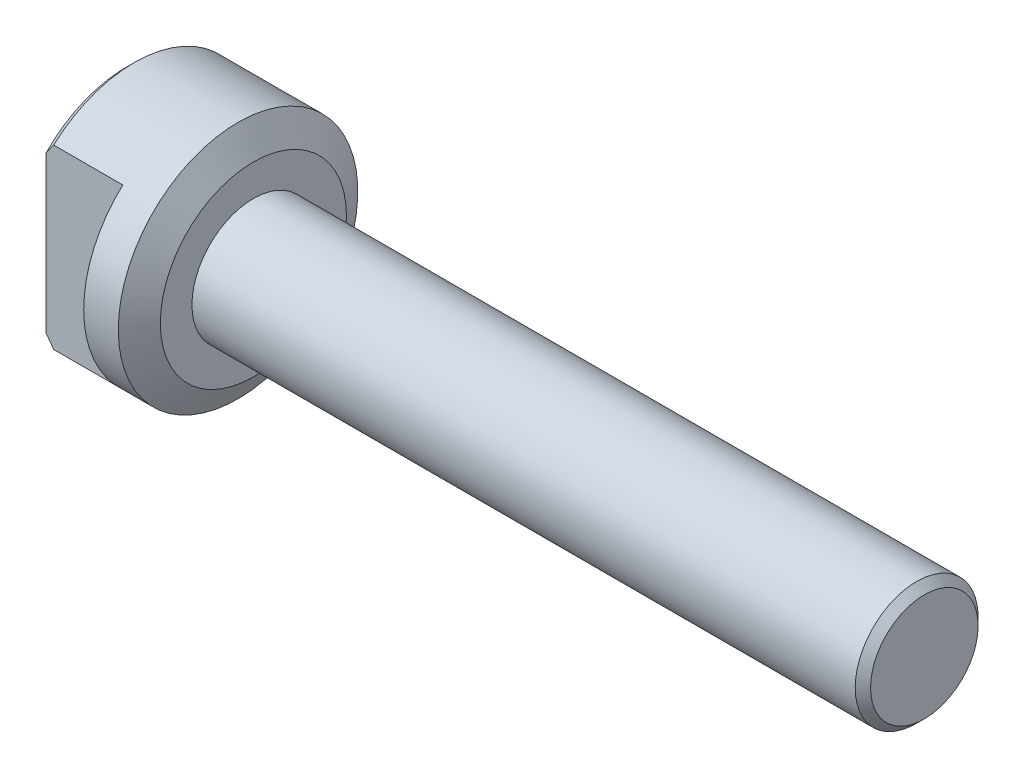
from build123d import *

# Parameters (mm, degrees)
CHAMFER1_SIZE      = 1
CHAMFER2_SIZE      = 1
SKETCH2_W          = 8.284694005
SKETCH2_H          = 60
SKETCH2_W_2        = 10.903172422
SKETCH2_H_2        = 30.692001108
CUT_EXTRUDE1_DEPTH = 10


with BuildPart() as part:
    # Sketch1 → Revolve1 (revolve)
    with BuildSketch(Plane.XY, mode=Mode.PRIVATE) as revolve1_sk:
        Polygon((-26.210699301, 0), (-26.210699301, 15.59), (-11.710699301, 15.59), (-9.710699301, 12.12), (-9.710699301, 8), (77.639300699, 8), (77.639300699, 0), align=None)
    revolve(revolve1_sk.sketch.rotate(Axis((-41.923036121, 0, 0), (1, 0, 0)), 90), axis=Axis((-41.923036121, 0, 0), (1, 0, 0)))

    # Chamfer1
    chamfer1_edges = [part.edges().sort_by_distance(p)[0] for p in [
        (-26.210699301, 0, -15.59),
    ]]
    chamfer(chamfer1_edges, length=CHAMFER1_SIZE)

    # Chamfer2
    chamfer2_edges = [part.edges().sort_by_distance(p)[0] for p in [
        (77.639300699, 0, -8),
    ]]
    chamfer(chamfer2_edges, length=CHAMFER2_SIZE)

    # Sketch2 → Cut-Extrude1 (cut)
    with BuildSketch(Plane.ZY.offset(26.210699301)):
        with Locations((-14.642347003, 15.254961706)):
            Rectangle(SKETCH2_W, SKETCH2_H)
        with Locations((15.951586211, 0.214629378)):
            Rectangle(SKETCH2_W_2, SKETCH2_H_2)
    extrude(amount=-CUT_EXTRUDE1_DEPTH, mode=Mode.SUBTRACT)


solid = part.part
